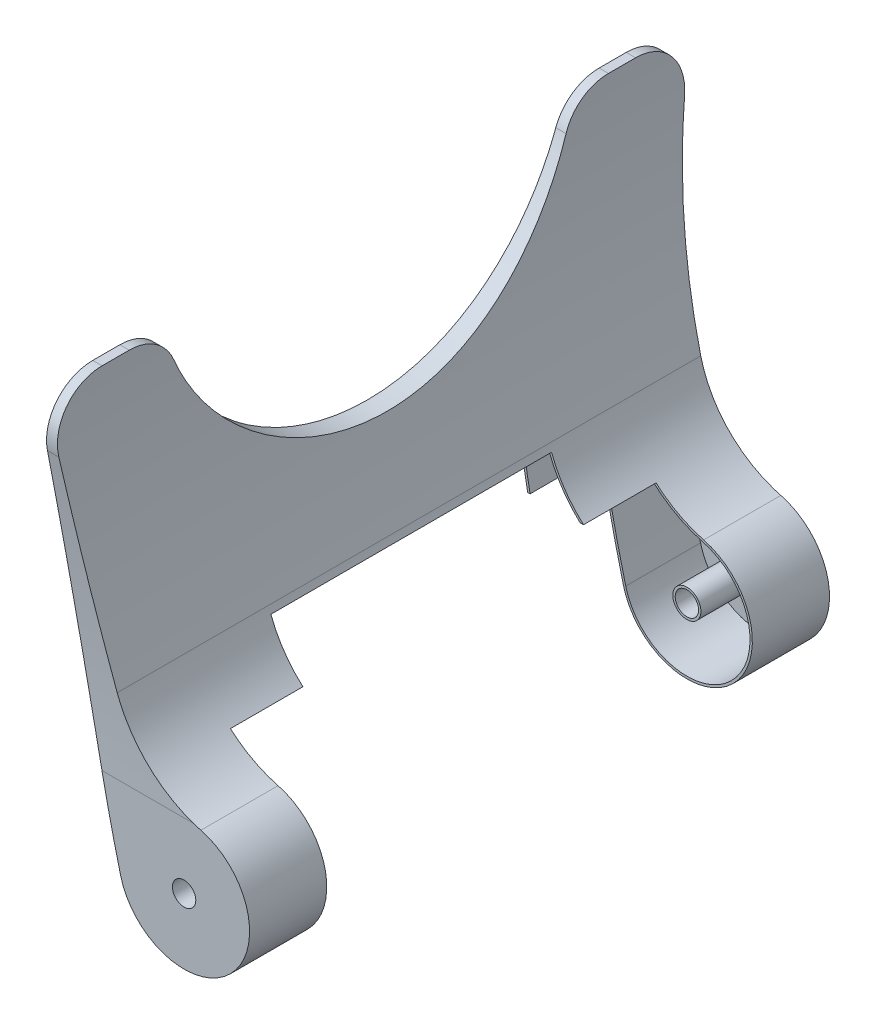
from build123d import *

# Parameters (mm, degrees)
BOSS_EXTRUDE1_DEPTH = 150
CUT_EXTRUDE5_DEPTH  = 101.5
SKETCH3_R           = 5
CUT_EXTRUDE6_DEPTH  = 277
CUT_EXTRUDE8_DEPTH  = 138.5
SHELL1_T            = -1


with BuildPart() as part:
    # Sketch1 → Boss-Extrude1 (new, symmetric)
    with BuildSketch(Plane.XY):
        with BuildLine():
            Line((-49, 168), (-45, 168))
            ThreePointArc((-45, 168), (-40.070744665, 113.846892769), (-27.842355225, 60.862715201))
            ThreePointArc((-27.842355225, 60.862715201), (-14.721546329, 39.414338757), (7.179487179, 27.063905185))
            ThreePointArc((7.179487179, 27.063905185), (19.713239873, -19.884370086), (-27.124948702, -6.945297538))
            ThreePointArc((-27.124948702, -6.945297538), (-43.592377915, 79.835895525), (-49, 168))
        make_face()
    extrude(amount=BOSS_EXTRUDE1_DEPTH, both=True)

    # Sketch2 → Cut-Extrude5 (cut, symmetric)
    with BuildSketch(Plane(origin=(0, 0, 0), x_dir=(0, 0, -1), z_dir=(1, 0, 0))):
        with BuildLine():
            ThreePointArc((-133.790691972, 144.666666667), (-129.345678345, 160.909944487), (-114.070426028, 168))
            Line((-114.070426028, 168), (-150, 168))
            Line((-150, 168), (-150, -28))
            Line((-150, -28), (-124, -28))
            Line((-124, -28), (-124, -8))
            Line((-124, -8), (-124, 28))
            ThreePointArc((-124, 28), (-126.451967382, 86.538382196), (-133.790691972, 144.666666667))
        make_face()
        with BuildLine():
            Line((102.46950766, 168), (-102.46950766, 168))
            ThreePointArc((-102.46950766, 168), (-91.187986163, 164.514456477), (-83.838688085, 155.272727273))
            ThreePointArc((-83.838688085, 155.272727273), (0, 98), (83.838688085, 155.272727273))
            ThreePointArc((83.838688085, 155.272727273), (91.187986163, 164.514456477), (102.46950766, 168))
        make_face()
        with BuildLine():
            Line((150, 168), (114.070426028, 168))
            ThreePointArc((114.070426028, 168), (129.345678345, 160.909944487), (133.790691972, 144.666666667))
            ThreePointArc((133.790691972, 144.666666667), (126.451967382, 86.538382196), (124, 28))
            Line((124, 28), (124, -8))
            Line((124, -8), (124, -28))
            Line((124, -28), (150, -28))
            Line((150, -28), (150, 168))
        make_face()
    extrude(amount=CUT_EXTRUDE5_DEPTH, both=True, mode=Mode.SUBTRACT)

    # Sketch3 → Cut-Extrude6 (cut)
    with BuildSketch(Plane.XY.offset(124)):
        Circle(SKETCH3_R)
    extrude(amount=-CUT_EXTRUDE6_DEPTH, mode=Mode.SUBTRACT)

    # Sketch4 → Cut-Extrude8 (cut, symmetric)
    with BuildSketch(Plane(origin=(0, 0, 0), x_dir=(0, 0, -1), z_dir=(1, 0, 0))):
        Polygon((-91, -28), (-91, 38), (-60, 38), (-60, 58), (60, 58), (60, 38), (91, 38), (91, -28), align=None)
    extrude(amount=CUT_EXTRUDE8_DEPTH, both=True, mode=Mode.SUBTRACT)

    # Shell1
    shell1_openings = [part.faces().sort_by_distance(p)[0] for p in [
        (-25.132161433, 38, 75.5),
        (-29.63441401, 47.053048744, 60),
        (-33.694776993, 58, 0),
        (-29.63441401, 47.053048744, -60),
        (-25.132161433, 38, -75.5),
        (-4.519844727, 5.226646447, 91),
        (-4.519844727, 5.226646447, -91),
    ]]
    offset(amount=SHELL1_T, openings=shell1_openings)


solid = part.part
